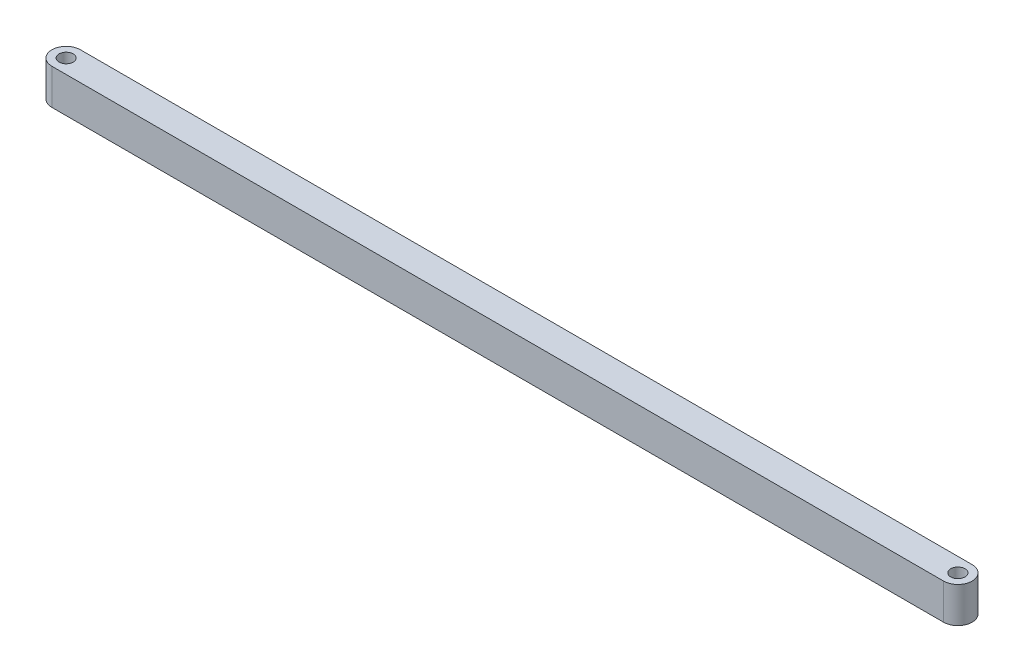
from build123d import *

# Parameters (mm, degrees)
SKETCH1_R           = 2
BOSS_EXTRUDE1_DEPTH = 10


with BuildPart() as part:
    # Sketch1 → Boss-Extrude1 (new body)
    with BuildSketch(Plane(origin=(0, 0, 0), x_dir=(1, 0, 0), z_dir=(0, 1, 0))):
        with BuildLine():
            Line((-125, 4), (125, 4))
            ThreePointArc((125, 4), (129, 0), (125, -4))
            Line((125, -4), (-125, -4))
            ThreePointArc((-125, -4), (-129, 0), (-125, 4))
        make_face()
        with Locations(Location((-125, 0, 0), (0, 0, 270))):
            Circle(SKETCH1_R, mode=Mode.SUBTRACT)
        with Locations(Location((125, 0, 0), (0, 0, 270))):
            Circle(SKETCH1_R, mode=Mode.SUBTRACT)
    extrude(amount=BOSS_EXTRUDE1_DEPTH)


solid = part.part
